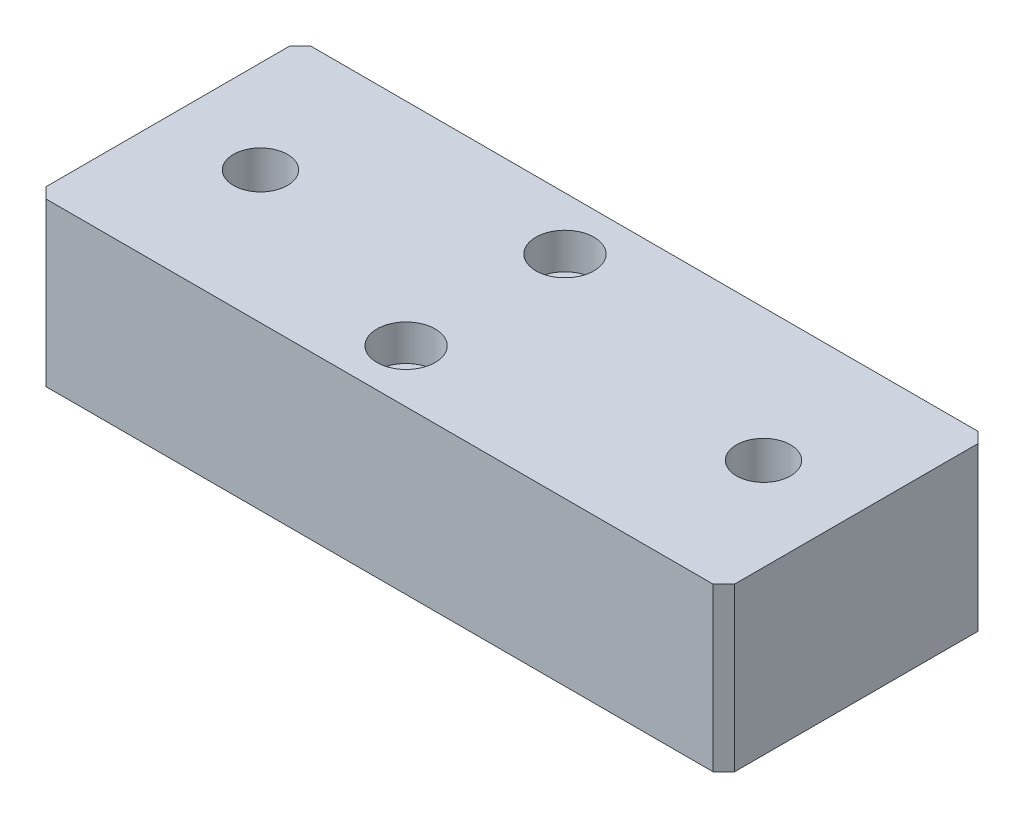
SolidWorks part; units mm, degrees
material "A6061"
ref_plane "前基準面" through (0, 0, 0) normal (0, 0, 1) x (1, 0, 0)
ref_plane "上基準面" through (0, 0, 0) normal (0, 1, 0) x (1, 0, 0)
ref_plane "右基準面" through (0, 0, 0) normal (1, 0, 0) x (0, 0, -1)
sketch "草图1" plane through (0, 0, 0) normal (0, 1, 0) x (1, 0, 0)
  line L1 (-65, -25) -> (65, -25)
  line L2 (-65, -25) -> (-65, 25)
  line L3 (-65, 25) -> (65, 25)
  line L4 (65, -25) -> (65, 25)
  line L5 (-65, -25) -> (65, 25) construction
  line L6 (-65, 25) -> (65, -25) construction
  point P0 (0, 0)
  dimension "D1" = 130
  dimension "D2" = 50
extrude "凸台-拉伸1" add sketch "草图1" along normal mid plane 30.7
chamfer "倒角1" distance 2 angle 45 4 edges at (65, 0, -25) (65, 0, 25) (-65, 0, -25) (-65, 0, 25)
hole_wizard "M12 螺纹孔1" positions "草图2" profile "草图3" tap size "M12" standard "GB" end condition through all
sketch "草图2" plane through (0, 15.35, 0) normal (0, 1, 0) x (1, 0, 0)
  line L0 (0, 39.2319) -> (0, 0) construction
  point P0 (-47.5, 0)
  point P8 (47.5, 0)
  dimension "D1" = 95
sketch "草图3" plane through (-47.5, 15.35, 0) normal (1, 0, 0) x (0, 0, 1)
  line L0 (0, 0) -> (0, 30.7)
  line L1 (0, 30.7) -> (5.1, 30.7)
  line L2 (5.1, 30.7) -> (5.1, 0)
  line L5 (5.1, 0) -> (0, 0)
  line L11 (0, -6.35) -> (0, 107.95) construction
  dimension "螺纹线主直径" = 10.2
  dimension "通孔螺纹孔钻头深度" = 30.7
hole_wizard "打孔尺寸(%根据)内六角圆柱头螺钉的类型1" positions "草图4" profile "草图5" counterbore size "M6" standard "GB" end condition through all
sketch "草图4" plane through (0, 15.35, 0) normal (0, 1, 0) x (1, 0, 0)
  line L2 (0, 0) -> (-34.3014, 0) construction
  line L4 (65, -23) -> (65, 23) construction
  point P0 (-5, -15)
  point P2 (-5, 15)
  dimension "D1" = 30
  dimension "D2" = 70
sketch "草图5" plane through (-5, 15.35, 15) normal (1, 0, 0) x (0, 0, 1)
  line L0 (0, 0) -> (0, 30.7)
  line L1 (0, 30.7) -> (3.3, 30.7)
  line L3 (3.3, 30.7) -> (3.3, 6.8)
  line L4 (3.3, 6.8) -> (5.5, 6.8)
  line L5 (5.5, 6.8) -> (5.5, 0)
  line L7 (5.5, 0) -> (0, 0)
  line L11 (0, -6.35) -> (0, 107.95) construction
  dimension "通孔孔直径" = 6.6
  dimension "通孔孔深度" = 30.7
  dimension "柱形沉头孔直径" = 11
  dimension "柱形沉头孔深度" = 6.8
